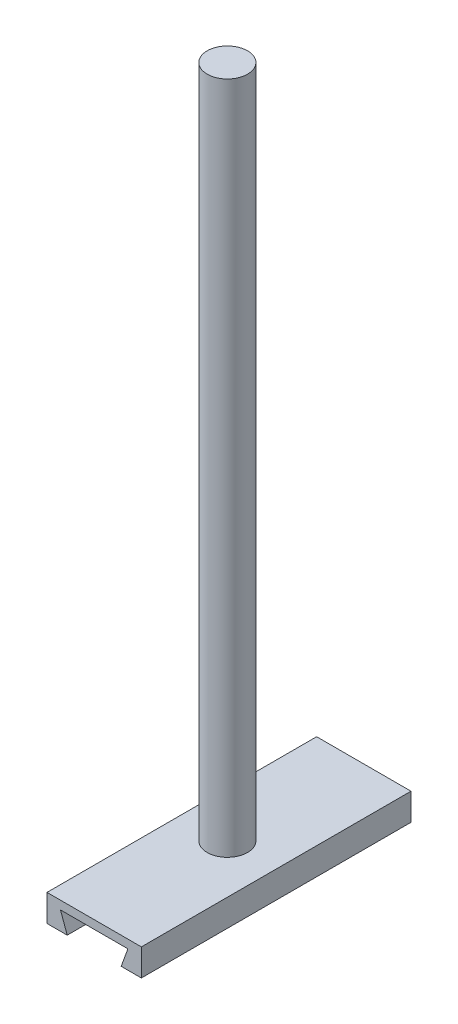
from build123d import *

# Parameters (mm, degrees)
BOSS_EXTRUDE1_DEPTH = 200
SKETCH2_R           = 15
BOSS_EXTRUDE2_DEPTH = 500


with BuildPart() as part:
    # Sketch1 → Boss-Extrude1 (new body)
    with BuildSketch(Plane.XY):
        Polygon((-30.262159038, 19.219105843), (39.737840962, 19.219105843), (39.737840962, -0.780894157), (24.737840962, -0.780894157), (29.737840962, 12.95649294), (-20.262159038, 12.95649294), (-15.262159038, -0.780894157), (-30.262159038, -0.780894157), align=None)
    extrude(amount=BOSS_EXTRUDE1_DEPTH)

    # Sketch2 → Boss-Extrude2 (add)
    with BuildSketch(Plane(origin=(0, 19.219105843, 0), x_dir=(1, 0, 0), z_dir=(0, 1, 0))):
        with Locations(Location((3.524411209, -100, 0), (0, 0, 90))):
            Circle(SKETCH2_R)
    extrude(amount=BOSS_EXTRUDE2_DEPTH)


solid = part.part
